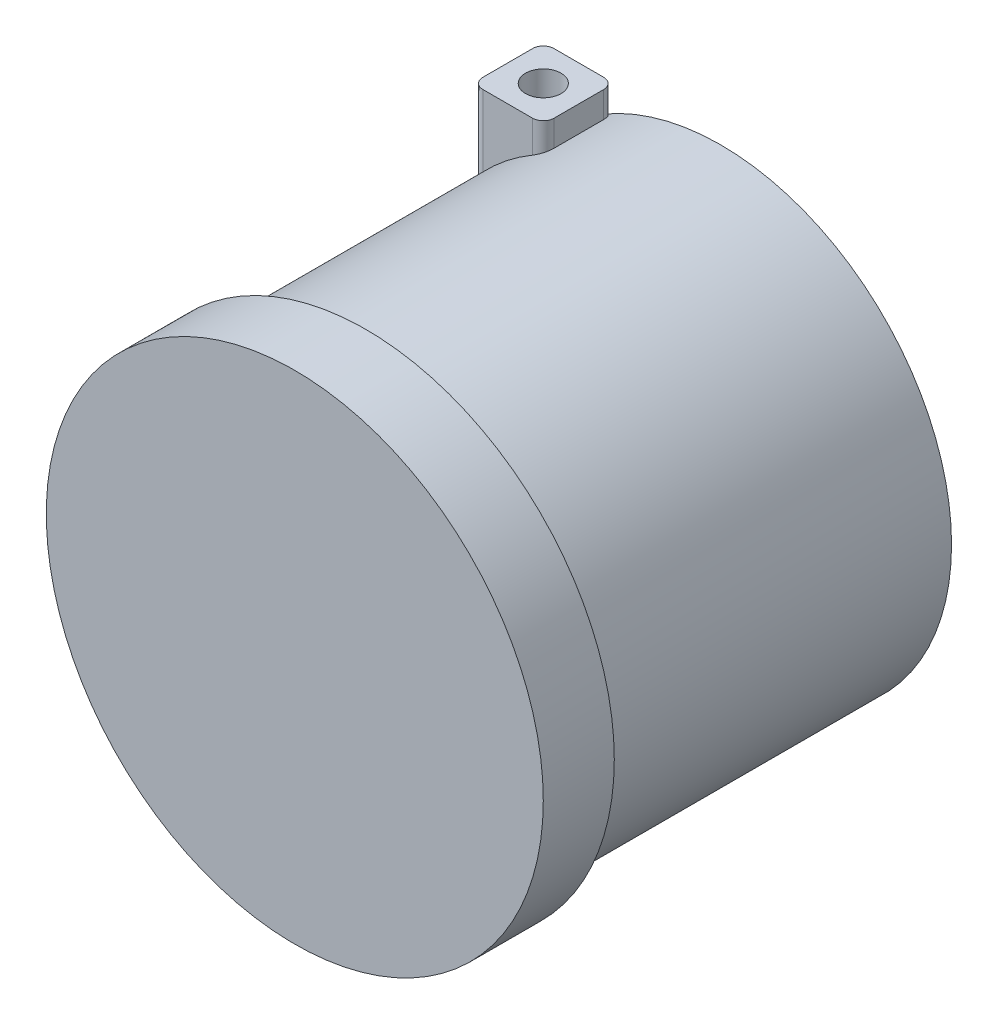
SolidWorks part; units mm, degrees
ref_plane "Front Plane" through (0, 0, 0) normal (0, 0, 1) x (1, 0, 0)
ref_plane "Top Plane" through (0, 0, 0) normal (0, 1, 0) x (1, 0, 0)
ref_plane "Right Plane" through (0, 0, 0) normal (1, 0, 0) x (0, 0, -1)
sketch "Sketch1" plane through (0, 0, 0) normal (0, 0, 1) x (1, 0, 0)
  circle A0 centre (0, 0) radius 65
  dimension "D1" = 130
extrude "Boss-Extrude1" add sketch "Sketch1" along normal blind 100
sketch "Sketch2" plane through (0, 0, 100) normal (0, 0, 1) x (1, 0, 0)
  circle A0 centre (0, 0) radius 70
  dimension "D1" = 140
extrude "Boss-Extrude2" add sketch "Sketch2" along normal blind 20 contours A0
sketch "Sketch4" plane through (0, 0, 0) normal (0, 0, -1) x (-1, 0, 0)
  line L1 (30, 40.911) -> (50, 40.911)
  line L2 (30, 40.911) -> (30, 65)
  line L3 (30, 65) -> (50, 65)
  line L4 (50, 40.911) -> (50, 65)
  dimension "D1" = 65
  dimension "D2" = 50
  dimension "D3" = 20
extrude "Boss-Extrude4" add sketch "Sketch4" against normal blind 20
sketch "Sketch5" plane through (0, 65, 0) normal (0, 1, 0) x (1, 0, 0)
  circle A0 centre (-40, -10) radius 5
extrude "Cut-Extrude1" cut sketch "Sketch5" against normal blind 15
fillet "Fillet1" radius 3 4 edges at (-30, 61.3314, 0) (-30, 61.3314, 20) (-50, 53.2666, 20) (-50, 53.2666, 0)
